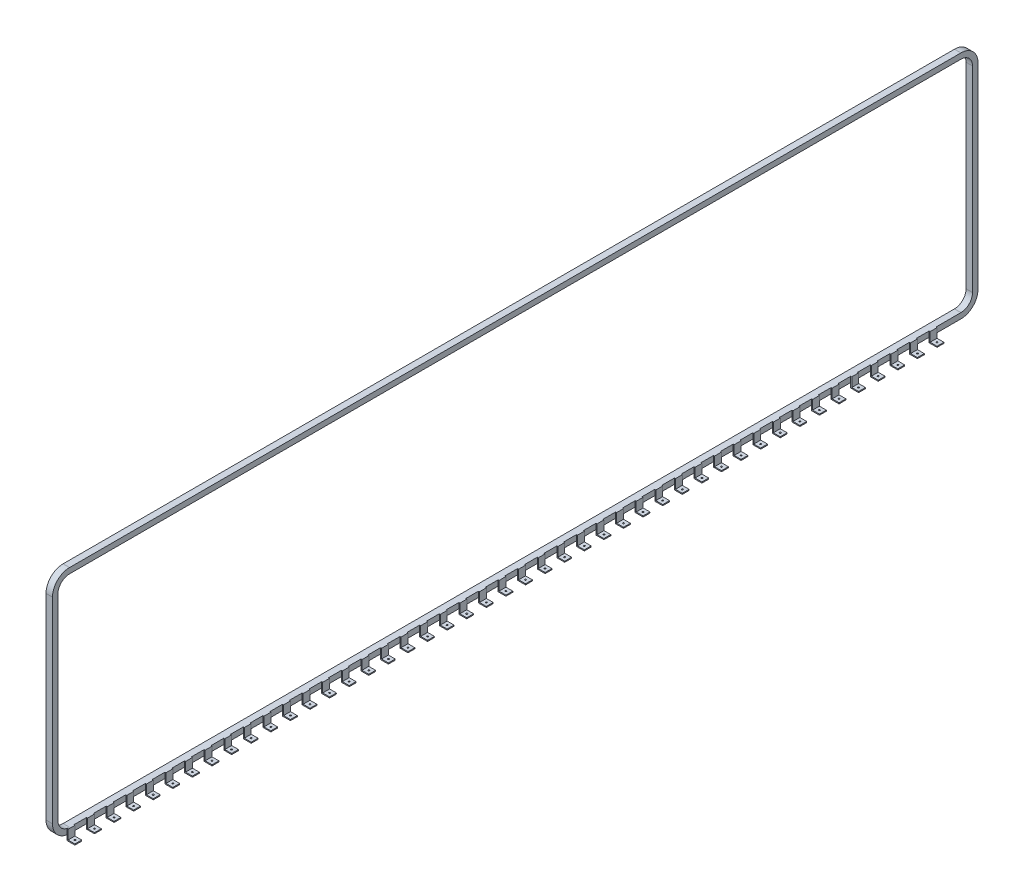
from build123d import *

# Parameters (mm, degrees)
EXTRUDE_1_DEPTH        = 18.8
SKETCH_2_W             = 20
SKETCH_2_H             = 30
EXTRUDE_1_2_DEPTH      = 3
SKETCH_3_W             = 20
SKETCH_3_H             = 3
EXTRUDE_2_DEPTH        = 20
HOLE_WIZARD_M5_1_D     = 4.2
PATTERN_LINEAR_1_COUNT = 45
PATTERN_LINEAR_1_PITCH = 57.15


with BuildPart() as part:
    # 草图1 → Extrude 1 (new body)
    with BuildSketch(Plane(origin=(0, 0, 0), x_dir=(0, 0, -1), z_dir=(1, 0, 0))):
        with BuildLine():
            Line((1349.81, 286.19), (1349.81, -286.19))
            ThreePointArc((1349.81, -286.19), (1335.220988771, -321.410988771), (1300, -336))
            Line((1300, -336), (-1300, -336))
            ThreePointArc((-1300, -336), (-1335.220988771, -321.410988771), (-1349.81, -286.19))
            Line((-1349.81, -286.19), (-1349.81, 286.19))
            ThreePointArc((-1349.81, 286.19), (-1335.220988771, 321.410988771), (-1300, 336))
            Line((-1300, 336), (1300, 336))
            ThreePointArc((1300, 336), (1335.220988771, 321.410988771), (1349.81, 286.19))
        make_face()
        with BuildLine():
            Line((1333.81, 286.19), (1333.81, -286.19))
            ThreePointArc((1333.81, -286.19), (1323.907280272, -310.097280272), (1300, -320))
            Line((1300, -320), (-1300, -320))
            ThreePointArc((-1300, -320), (-1323.907280272, -310.097280272), (-1333.81, -286.19))
            Line((-1333.81, -286.19), (-1333.81, 286.19))
            ThreePointArc((-1333.81, 286.19), (-1323.907280272, 310.097280272), (-1300, 320))
            Line((-1300, 320), (1300, 320))
            ThreePointArc((1300, 320), (1323.907280272, 310.097280272), (1333.81, 286.19))
        make_face(mode=Mode.SUBTRACT)
    extrude(amount=EXTRUDE_1_DEPTH)

    # 草图2 → Extrude 1 2 (add)
    with BuildSketch(Plane(origin=(18.8, 0, 0), x_dir=(0, 0, -1), z_dir=(1, 0, 0))):
        with Locations((-1297.35, -335)):
            Rectangle(SKETCH_2_W, SKETCH_2_H)
    extrude_1_2 = extrude(amount=EXTRUDE_1_2_DEPTH)

    # 草图3 → 凸台-拉伸2 (add)
    with BuildSketch(Plane(origin=(21.8, 0, 0), x_dir=(0, 0, -1), z_dir=(1, 0, 0))):
        with Locations((-1297.35, -348.5)):
            Rectangle(SKETCH_3_W, SKETCH_3_H)
    extrude_2 = extrude(amount=EXTRUDE_2_DEPTH)

    # M5 螺纹孔1 (through all)
    with Locations(Plane(origin=(0, -350, 0), x_dir=(-1, 0, 0), z_dir=(0, -1, 0))):
        with Locations((-31.8, -1297.35)):
            hole_wizard_m5_1 = Hole(HOLE_WIZARD_M5_1_D / 2)

    # 阵列(线性)1: Extrude 1 2, 凸台-拉伸2, M5 螺纹孔1 ×45
    with Locations(*[(0, 0, -i * PATTERN_LINEAR_1_PITCH) for i in range(1, PATTERN_LINEAR_1_COUNT)]):
        add(extrude_1_2)
        add(extrude_2)
        add(hole_wizard_m5_1, mode=Mode.SUBTRACT)


solid = part.part
